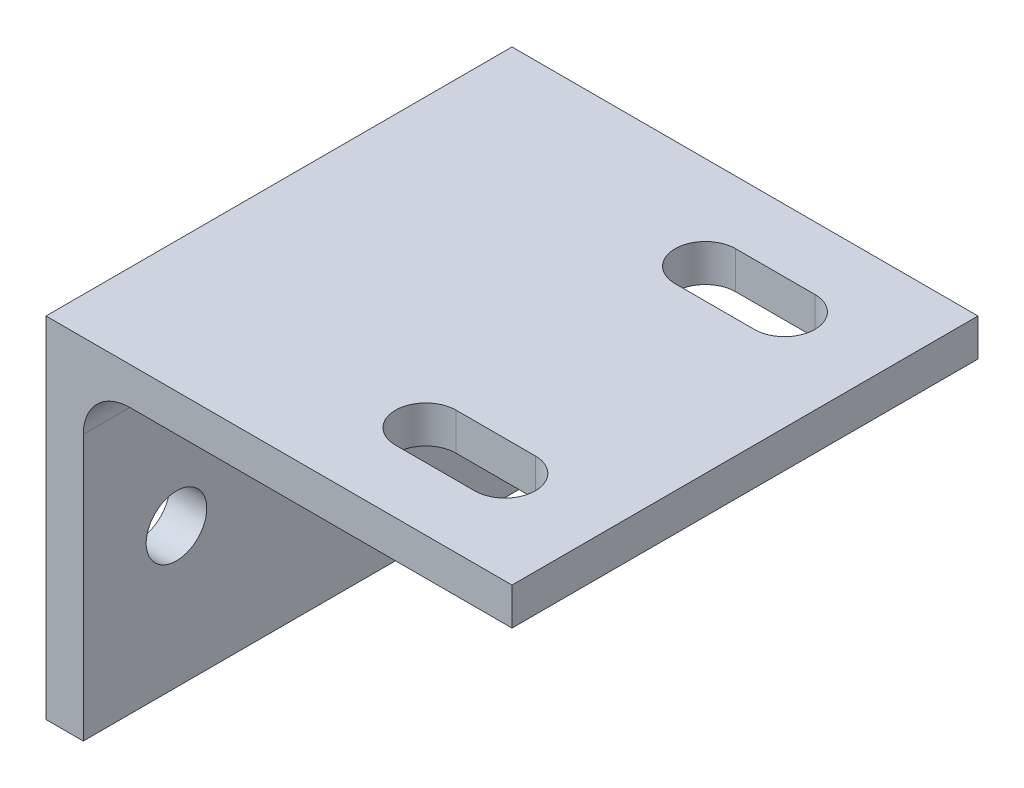
from build123d import *

# Parameters (mm, degrees)
EXTRUDE_1_DEPTH     = 100
CUT_EXTRUDE_1_DEPTH = 100
SKETCH_3_R          = 6.5
CUT_EXTRUDE_2_DEPTH = 100
FILLET_1_R          = 10


with BuildPart() as part:
    # 草图1 → 凸台-拉伸1 (new body)
    with BuildSketch(Plane.XY):
        Polygon((0, 0), (-100, 0), (-100, -75), (-92, -75), (-92, -8), (0, -8), align=None)
    extrude(amount=EXTRUDE_1_DEPTH)

    # 草图2 → 切除-拉伸1 (cut)
    with BuildSketch(Plane(origin=(0, 0, 0), x_dir=(1, 0, 0), z_dir=(0, 1, 0))):
        with BuildLine():
            Line((-38.5, -13.5), (-21.5, -13.5))
            ThreePointArc((-21.5, -13.5), (-15, -20), (-21.5, -26.5))
            Line((-21.5, -26.5), (-38.5, -26.5))
            ThreePointArc((-38.5, -26.5), (-45, -20), (-38.5, -13.5))
        make_face()
        with BuildLine():
            Line((-38.5, -73.5), (-21.5, -73.5))
            ThreePointArc((-21.5, -73.5), (-15, -80), (-21.5, -86.5))
            Line((-21.5, -86.5), (-38.5, -86.5))
            ThreePointArc((-38.5, -86.5), (-45, -80), (-38.5, -73.5))
        make_face()
    extrude(amount=-CUT_EXTRUDE_1_DEPTH, mode=Mode.SUBTRACT)

    # 草图3 → 切除-拉伸2 (cut)
    with BuildSketch(Plane(origin=(-92, 0, 0), x_dir=(0, 0, -1), z_dir=(1, 0, 0))):
        with Locations((-80, -45)):
            Circle(SKETCH_3_R)
        with Locations((-20, -45)):
            Circle(SKETCH_3_R)
    extrude(amount=-CUT_EXTRUDE_2_DEPTH, mode=Mode.SUBTRACT)

    # 圆角1
    fillet_1_edges = [part.edges().sort_by_distance(p)[0] for p in [
        (-92, -8, 50),
    ]]
    fillet(fillet_1_edges, radius=FILLET_1_R)


solid = part.part
